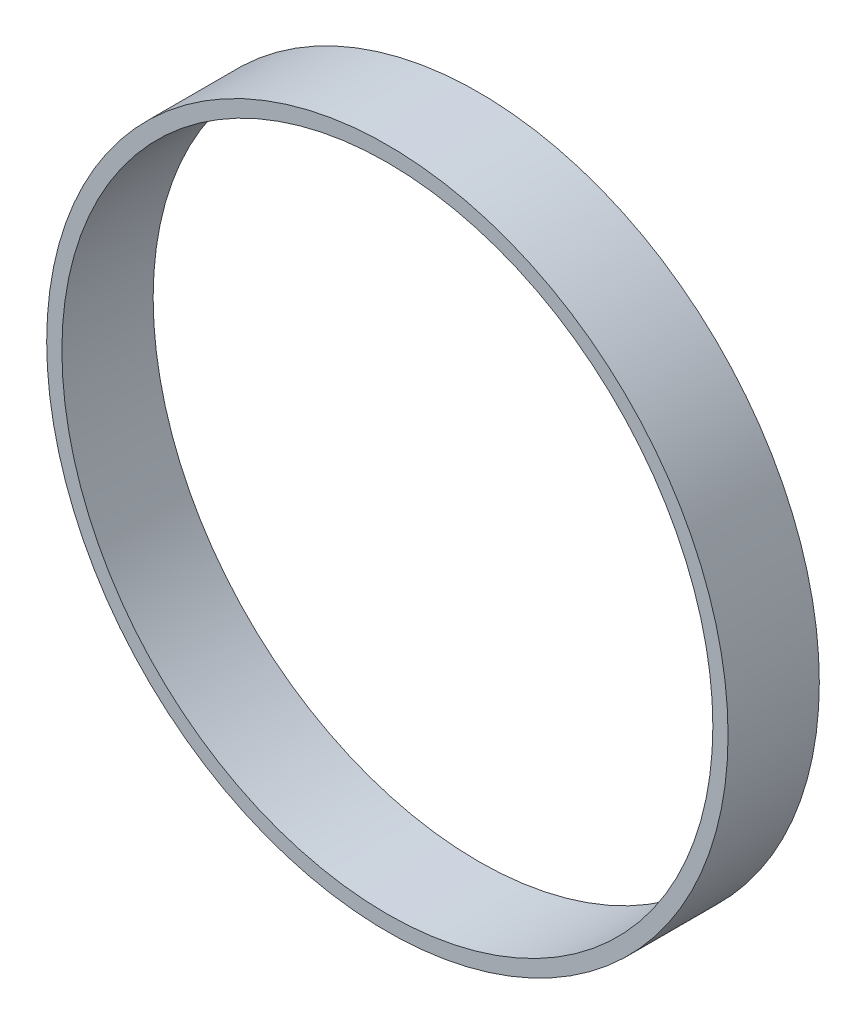
from build123d import *

# Parameters (mm, degrees)
SKETCH1_R           = 56
SKETCH1_R_2         = 53.5
BOSS_EXTRUDE1_DEPTH = 15


with BuildPart() as part:
    # Sketch1 → Boss-Extrude1 (new body)
    with BuildSketch(Plane.XY):
        Circle(SKETCH1_R)
        Circle(SKETCH1_R_2, mode=Mode.SUBTRACT)
    extrude(amount=BOSS_EXTRUDE1_DEPTH)


solid = part.part
